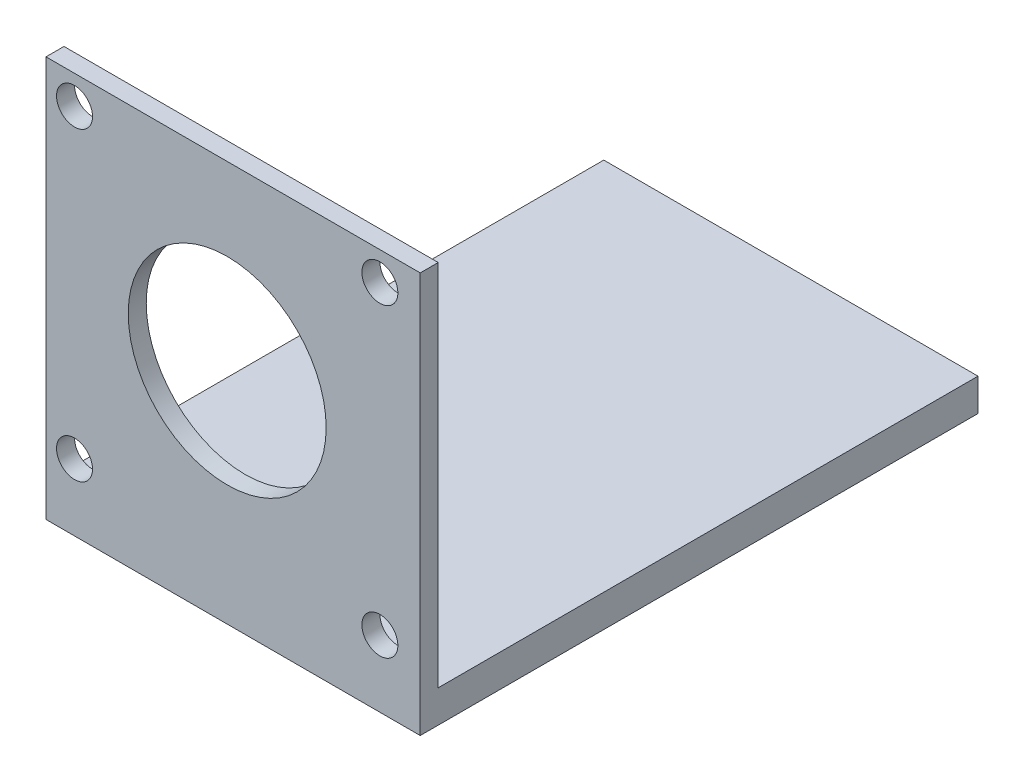
SolidWorks part; units mm, degrees
material "1060 合金"
ref_plane "前视基准面" through (0, 0, 0) normal (0, 0, 1) x (1, 0, 0)
ref_plane "上视基准面" through (0, 0, 0) normal (0, 1, 0) x (1, 0, 0)
ref_plane "右视基准面" through (0, 0, 0) normal (1, 0, 0) x (0, 0, -1)
other "Configuration Table"
sketch "草图1" plane through (0, 0, 0) normal (0, 0, 1) x (1, 0, 0)
  line L0 (-50.3546, -47.2658) -> (-50.3546, -53.6454)
  line L2 (-50.3546, -47.2658) -> (-50.3546, 50.3546)
  line L3 (-50.3546, 50.3546) -> (53.6454, 50.3546)
  line L4 (53.6454, -53.6454) -> (53.6454, 50.3546)
  line L5 (-50.3546, -47.2658) -> (53.6454, 50.3546) construction
  line L6 (-50.3546, 50.3546) -> (53.6454, -53.6454) construction
  line L10 (-50.3546, -53.6454) -> (-50.3546, -60.9954)
  line L11 (-50.3546, -60.9954) -> (53.6454, -60.9954)
  line L12 (53.6454, -60.9954) -> (53.6454, -53.6454)
  point P0 (0, 0)
  dimension "D1" = 104
  dimension "D2" = 104
  dimension "D3" = 7.35
extrude "凸台-拉伸1" add sketch "草图1" along normal blind 5
sketch "草图4" plane through (0, 0, 5) normal (0, 0, 1) x (1, 0, 0)
  circle A0 centre (0, 0) radius 27.5
  dimension "D1" = 55
extrude "切除-拉伸4" cut sketch "草图4" against normal blind 20
sketch "草图5" plane through (0, 0, 0) normal (0, 0, -1) x (-1, 0, 0)
  line L0 (50.3546, 50.3546) -> (50.3546, -60.9954) construction
  line L1 (-53.6454, -60.9954) -> (50.3546, -60.9954)
  line L2 (-53.6454, -60.9954) -> (-53.6454, -51.9954)
  line L3 (-53.6454, -51.9954) -> (50.3546, -51.9954)
  line L4 (50.3546, -60.9954) -> (50.3546, -51.9954)
  dimension "D1" = 9
extrude "凸台-拉伸2" add sketch "草图5" along normal blind 150
sketch "草图6" plane through (0, 0, 0) normal (0, 0, -1) x (-1, 0, 0)
  circle A0 centre (-42.4264, 42.4264) radius 5
  circle A1 centre (42.4264, 42.4264) radius 5
  circle A2 centre (42.4264, -42.4264) radius 5
  circle A3 centre (-42.4264, -42.4264) radius 5
  dimension "D1" = 10
extrude "切除-拉伸5" cut sketch "草图6" against normal through all both and the other way through all
